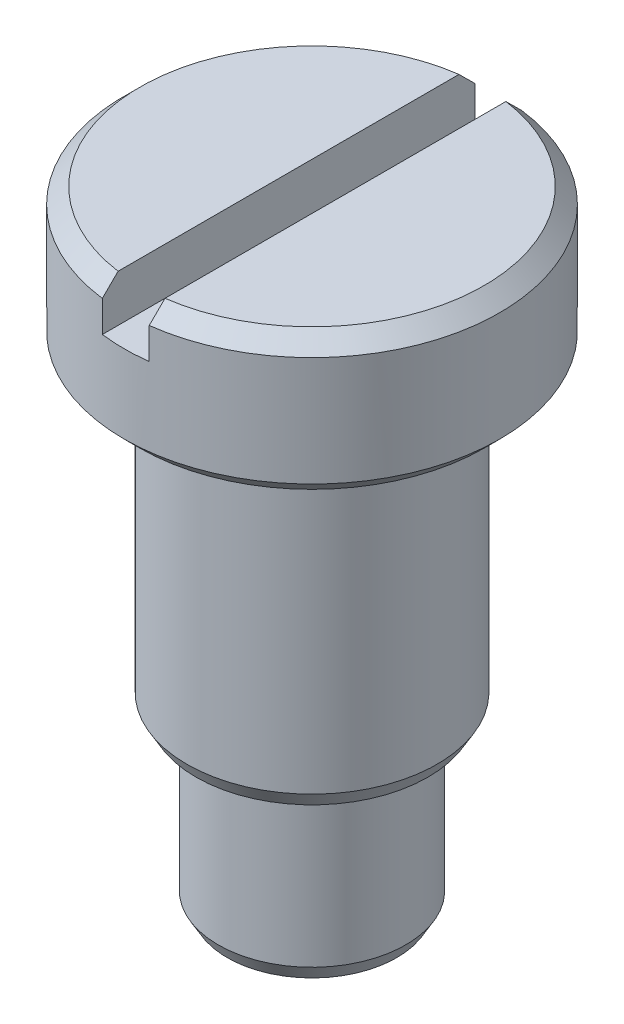
SolidWorks part; units mm, degrees
ref_plane "Front Plane" through (0, 0, 0) normal (0, 0, 1) x (1, 0, 0)
ref_plane "Top Plane" through (0, 0, 0) normal (0, 1, 0) x (1, 0, 0)
ref_plane "Right Plane" through (0, 0, 0) normal (1, 0, 0) x (0, 0, -1)
sketch "Sketch1" plane through (0, 0, 0) normal (0, 0, 1) x (1, 0, 0)
  line L0 (0, 0) -> (0, 40)
  line L1 (0, 0) -> (0, 40) construction
  line L3 (0, 40) -> (12, 40)
  line L4 (12, 40) -> (12, 31)
  line L5 (12, 31) -> (8, 31)
  line L6 (8, 31) -> (8, 11)
  line L7 (8, 11) -> (6, 11)
  line L10 (6, 11) -> (6, 0)
  line L11 (6, 0) -> (0, 0)
  point P1 (0.2062, 40)
  dimension "D1" = 11
  dimension "D2" = 31
  dimension "D3" = 6
  dimension "D5" = 40
  dimension "D7" = 8
  dimension "D8" = 12
revolve "Revolve1" add sketch "Sketch1" angle 360 about L1
chamfer "Chamfer1" distance 1 angle 45 2 edges at (0, 40, -12) (0, 31, -12)
chamfer "Chamfer2" distance 1 angle 30 2 edges at (0, 0, -6) (0, 11, -8)
cosmetic thread "Cosmetic Thread1" parameters "D1"=8, "D2"=10.072
sketch "Sketch2" plane through (0, 40, 0) normal (0, 1, 0) x (1, 0, 0)
  line L1 (-1.5, -15.2942) -> (1.5, -15.2942)
  line L2 (-1.5, -15.2942) -> (-1.5, 15.2942)
  line L3 (-1.5, 15.2942) -> (1.5, 15.2942)
  line L4 (1.5, -15.2942) -> (1.5, 15.2942)
  line L5 (-1.5, -15.2942) -> (1.5, 15.2942) construction
  line L6 (-1.5, 15.2942) -> (1.5, -15.2942) construction
  point P0 (0, 0)
  dimension "D1" = 3
extrude "Cut-Extrude1" cut sketch "Sketch2" against normal blind 3
